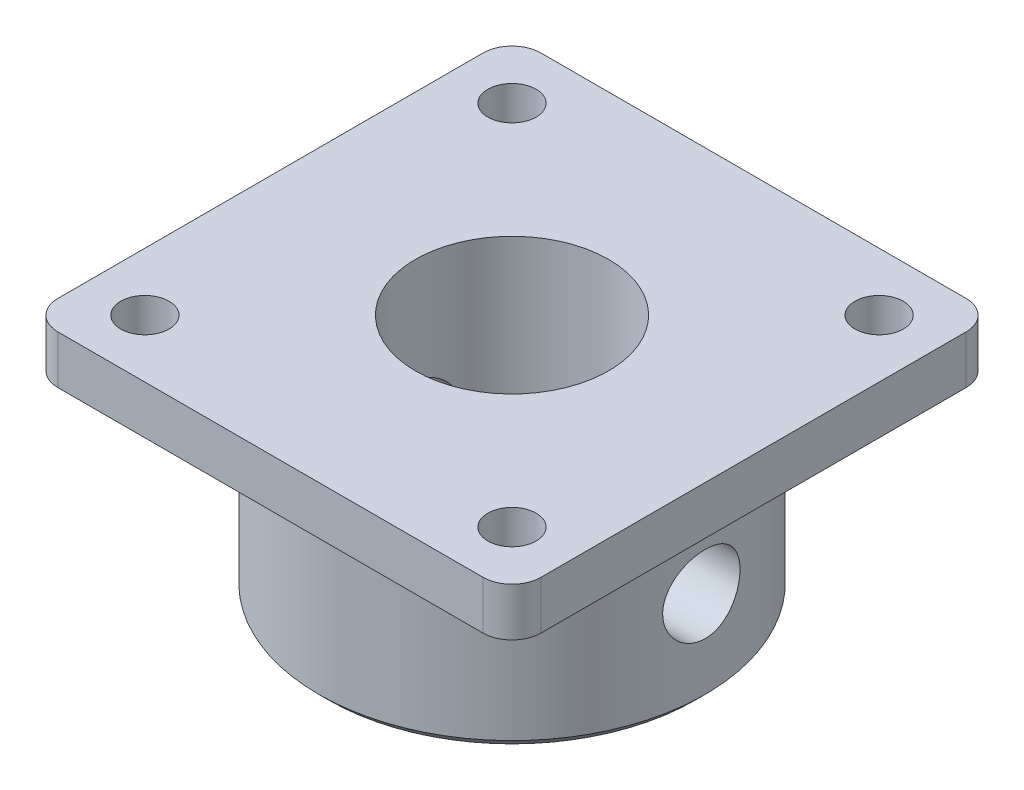
from build123d import *

# Parameters (mm, degrees)
SKETCH1_R               = 20
BOSS_EXTRUDE1_DEPTH     = 20
CUT_EXTRUDE5_DEPTH      = 25
CUT_EXTRUDE5_DEPTH_BACK = 25
SKETCH8_R               = 4
SKETCH9_W               = 50
SKETCH9_H               = 50
BOSS_EXTRUDE3_DEPTH     = 5
SKETCH10_R              = 10
CUT_EXTRUDE6_DEPTH      = 25
SKETCH11_R              = 2.5
CUT_EXTRUDE7_DEPTH      = 10
FILLET1_R               = 3
FILLET2_R               = 1
CHAMFER1_SIZE           = 1


with BuildPart() as part:
    # Sketch1 → Boss-Extrude1 (new body)
    with BuildSketch(Plane(origin=(0, 0, 0), x_dir=(1, 0, 0), z_dir=(0, 1, 0))):
        with Locations(Location((0, 0, 0), (0, 0, 270))):
            Circle(SKETCH1_R)
    extrude(amount=BOSS_EXTRUDE1_DEPTH)

    # Sketch8 → Cut-Extrude5 (cut, two sides: drawn at the far end of the back side and taken through both)
    with BuildSketch(Plane(origin=(0, 0, 0), x_dir=(0, 0, -1), z_dir=(1, 0, 0)).offset(-CUT_EXTRUDE5_DEPTH_BACK)):
        with Locations(Location((0, 10, 0), (0, 0, 180))):
            Circle(SKETCH8_R)
    extrude(amount=CUT_EXTRUDE5_DEPTH + CUT_EXTRUDE5_DEPTH_BACK, mode=Mode.SUBTRACT)

    # Sketch9 → Boss-Extrude3 (add)
    with BuildSketch(Plane(origin=(0, 20, 0), x_dir=(1, 0, 0), z_dir=(0, 1, 0))):
        Rectangle(SKETCH9_W, SKETCH9_H)
    extrude(amount=BOSS_EXTRUDE3_DEPTH)

    # Sketch10 → Cut-Extrude6 (cut)
    with BuildSketch(Plane(origin=(0, 25, 0), x_dir=(1, 0, 0), z_dir=(0, 1, 0))):
        with Locations(Location((0, 0, 0), (0, 0, 270))):
            Circle(SKETCH10_R)
    extrude(amount=-CUT_EXTRUDE6_DEPTH, mode=Mode.SUBTRACT)

    # Sketch11 → Cut-Extrude7 (cut)
    with BuildSketch(Plane(origin=(0, 25, 0), x_dir=(1, 0, 0), z_dir=(0, 1, 0))):
        with Locations(Location((-19, 19, 0), (0, 0, 270))):
            Circle(SKETCH11_R)
        with Locations(Location((-19, -19, 0), (0, 0, 270))):
            Circle(SKETCH11_R)
        with Locations(Location((19, -19, 0), (0, 0, 270))):
            Circle(SKETCH11_R)
        with Locations(Location((19, 19, 0), (0, 0, 270))):
            Circle(SKETCH11_R)
    extrude(amount=-CUT_EXTRUDE7_DEPTH, mode=Mode.SUBTRACT)

    # Fillet1
    fillet1_edges = [part.edges().sort_by_distance(p)[0] for p in [
        (25, 22.5, 25),
        (25, 22.5, -25),
        (-25, 22.5, -25),
        (-25, 22.5, 25),
    ]]
    fillet(fillet1_edges, radius=FILLET1_R)

    # Fillet2
    fillet2_edges = [part.edges().sort_by_distance(p)[0] for p in [
        (0, 20, -20),
    ]]
    fillet(fillet2_edges, radius=FILLET2_R)

    # Chamfer1
    chamfer1_edges = [part.edges().sort_by_distance(p)[0] for p in [
        (0, 0, -20),
        (0, 0, -10),
    ]]
    chamfer(chamfer1_edges, length=CHAMFER1_SIZE)


solid = part.part
